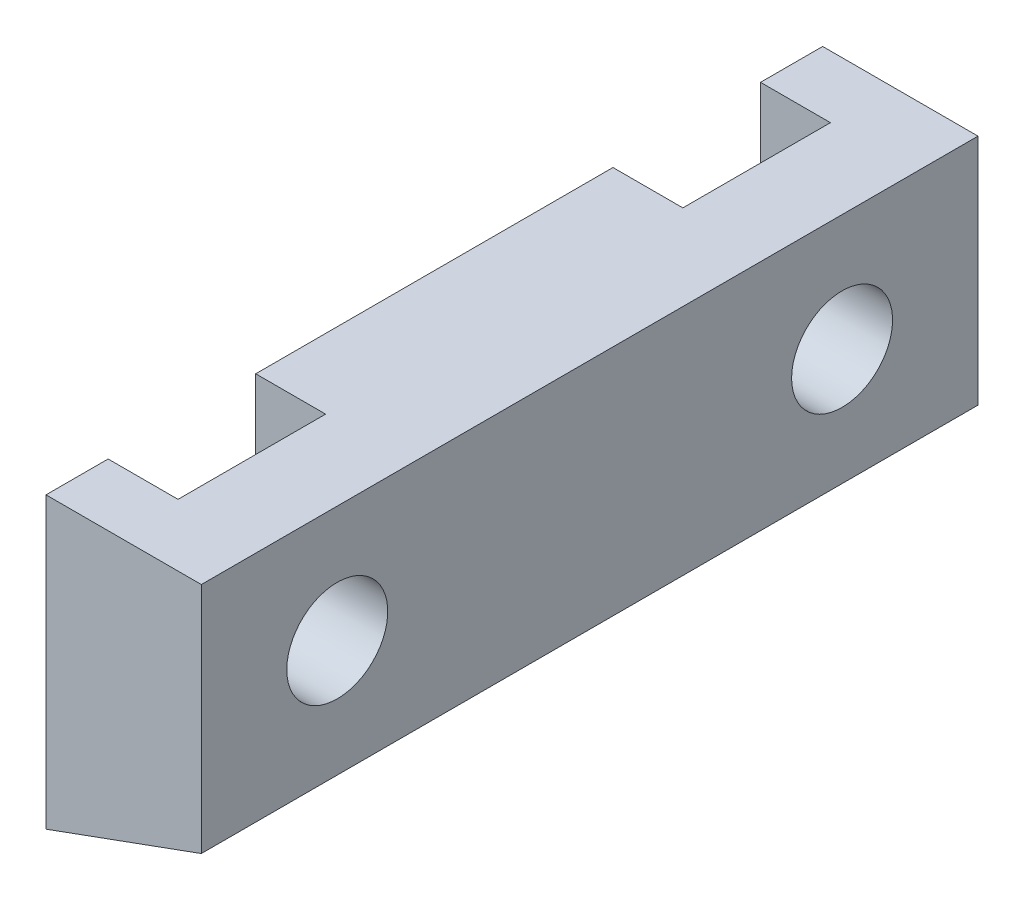
SolidWorks part; units mm, degrees
material "Q235-A"
ref_plane "Front Plane" through (0, 0, 0) normal (0, 0, 1) x (1, 0, 0)
ref_plane "Top Plane" through (0, 0, 0) normal (0, 1, 0) x (1, 0, 0)
ref_plane "Right Plane" through (0, 0, 0) normal (1, 0, 0) x (0, 0, -1)
sketch "Sketch2" plane through (0, 0, 0) normal (0, 0, 1) x (1, 0, 0)
  line L0 (0, 0) -> (0, 74.5588)
  line L1 (0, 74.5588) -> (40, 74.5588)
  line L2 (40, 74.5588) -> (40, 14.5588)
  line L3 (40, 14.5588) -> (0, 0)
  line L4 (0, 0) -> (54.1858, 0) construction
  dimension "D1" = 40
  dimension "D2" = 20
  dimension "D3" = 60
extrude "Boss-Extrude1" add sketch "Sketch2" along normal mid plane 200
sketch "Sketch3" plane through (0, 0, 0) normal (-1, 0, 0) x (0, 0, 1)
  line L0 (0, 0) -> (0, 99.5141) construction
  line L1 (100, 74.5588) -> (-100, 74.5588) construction
  line L2 (-46, -16.6564) -> (-84, -16.6564)
  line L3 (-46, -16.6564) -> (-46, 105.774)
  line L4 (-46, 105.774) -> (-84, 105.774)
  line L5 (-84, -16.6564) -> (-84, 105.774)
  line L6 (-46, -16.6564) -> (-84, 105.774) construction
  line L7 (-46, 105.774) -> (-84, -16.6564) construction
  line L8 (-100, 74.5588) -> (-100, 0) construction
  point P3 (-65, 44.5588)
  dimension "D1" = 38
  dimension "D2" = 30
  dimension "D3" = 35
extrude "Cut-Extrude1" cut sketch "Sketch3" against normal blind 18
mirror "Mirror1" about plane through (0, 0, 0) normal (0, 0, 1) of "Cut-Extrude1"
sketch "Sketch4" plane through (0, 0, 0) normal (1, 0, 0) x (0, 0, -1)
  line L0 (0, 0) -> (0, 44.5588) construction
  line L2 (-46, 74.5588) -> (46, 74.5588) construction
  line L3 (-65, 44.5588) -> (65, 44.5588) construction
  circle A0 centre (65, 44.5588) radius 13
  circle A1 centre (-65, 44.5588) radius 13
  point P8 (0, 44.5588)
  dimension "D3" = 26
  dimension "D1" = 30
  dimension "D2" = 130
extrude "Cut-Extrude2" cut sketch "Sketch4" along normal blind 60
